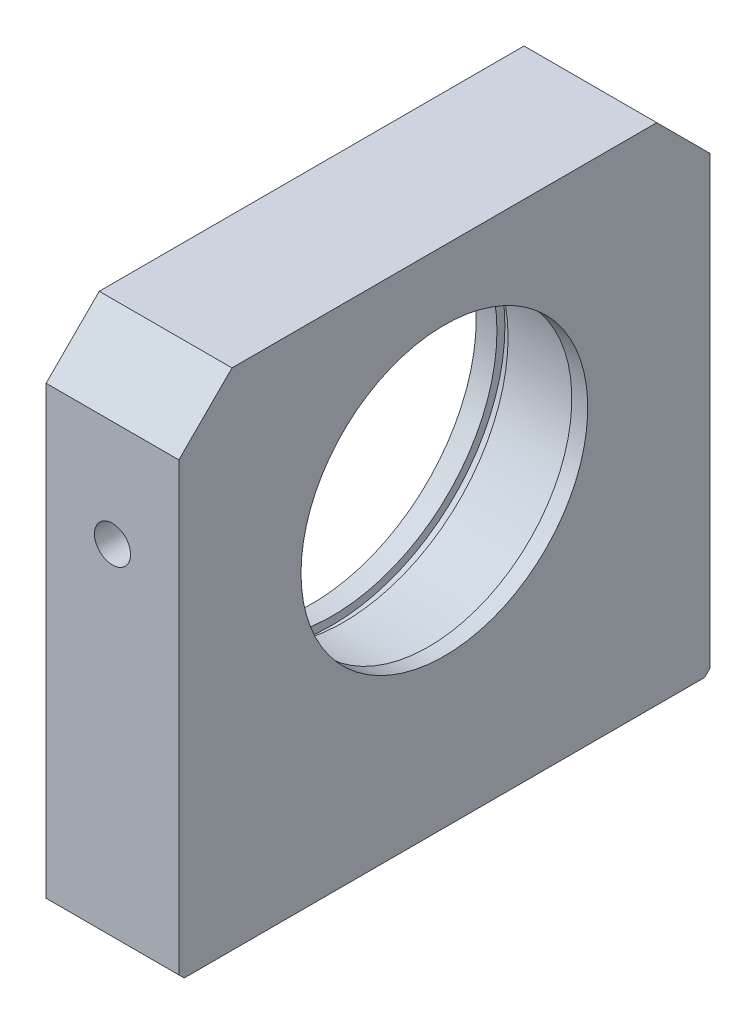
SolidWorks part; units mm, degrees
material "45#"
ref_plane "前基準面" through (0, 0, 0) normal (0, 0, 1) x (1, 0, 0)
ref_plane "上基準面" through (0, 0, 0) normal (0, 1, 0) x (1, 0, 0)
ref_plane "右基準面" through (0, 0, 0) normal (1, 0, 0) x (0, 0, -1)
sketch "草图1" plane through (0, 0, 0) normal (1, 0, 0) x (0, 0, -1)
  line L1 (-50, 47.5) -> (50, 47.5)
  line L2 (-50, 47.5) -> (-50, -47.5)
  line L3 (-50, -47.5) -> (50, -47.5)
  line L4 (50, 47.5) -> (50, -47.5)
  line L5 (-50, 47.5) -> (50, -47.5) construction
  line L6 (-50, -47.5) -> (50, 47.5) construction
  point P0 (0, 0)
  dimension "D1" = 95
  dimension "D2" = 100
extrude "凸台-拉伸1" add sketch "草图1" along normal blind 25
sketch "草图2" plane through (0, 0, 0) normal (-1, 0, 0) x (0, 0, 1)
  line L0 (0, 0) -> (0, 72.9224) construction
  line L1 (-50, 47.5) -> (50, 47.5) construction
  circle A0 centre (0, 7.5) radius 31
  dimension "D1" = 62
  dimension "D2" = 40
extrude "切除-拉伸1" cut sketch "草图2" against normal blind 22
sketch "草图3" plane through (22, 0, 0) normal (-1, 0, 0) x (0, 0, 1)
  circle A0 centre (0, 7.5) radius 27
  dimension "D1" = 54
extrude "切除-拉伸2" cut sketch "草图3" against normal through all
sketch "草图4" plane through (22, 0, 0) normal (-1, 0, 0) x (0, 0, 1)
  circle A0 centre (0, 7.5) radius 32.5
  dimension "D1" = 65
extrude "切除-拉伸3" cut sketch "草图4" along normal blind 2.1 from offset 16
hole_wizard "M8 螺纹孔1" positions "草图5" profile "草图6" tap size "M8" standard "GB"
sketch "草图5" plane through (0, 0, 50) normal (0, 0, 1) x (1, 0, 0)
  line L0 (12.5, 47.5) -> (12.5, -25.3343) construction
  line L1 (25, 47.5) -> (0, 47.5) construction
  point P0 (12.5, 17.5)
  dimension "D1" = 30
sketch "草图6" plane through (12.5, 17.5, 50) normal (1, 0, 0) x (0, -1, 0)
  line L0 (0, 0) -> (0, 17.7929)
  line L1 (0, 17.7929) -> (3.4, 15.75)
  line L2 (3.4, 15.75) -> (3.4, 0)
  line L5 (3.4, 0) -> (0, 0)
  line L10 (0, 17.7929) -> (-3.4, 15.75) construction
  line L11 (0, -6.35) -> (0, 107.95) construction
  dimension "螺纹孔钻头直径" = 6.8
  dimension "螺纹孔钻头深度" = 15.75
  dimension "导头角度" = 118
cosmetic thread "孔螺蚊线1" parameters "D1"=12, "D2"=8
hole_wizard "M8 螺纹孔2" positions "草图7" profile "草图8" tap size "M8" standard "GB"
sketch "草图7" plane through (0, 0, -50) normal (0, 0, -1) x (-1, 0, 0)
  point P0 (-12.5, 17.5)
sketch "草图8" plane through (12.5, 17.5, -50) normal (1, 0, 0) x (0, 1, 0)
  line L0 (0, 0) -> (0, 17.7929)
  line L1 (0, 17.7929) -> (3.4, 15.75)
  line L2 (3.4, 15.75) -> (3.4, 0)
  line L5 (3.4, 0) -> (0, 0)
  line L10 (0, 17.7929) -> (-3.4, 15.75) construction
  line L11 (0, -6.35) -> (0, 107.95) construction
  dimension "螺纹孔钻头直径" = 6.8
  dimension "螺纹孔钻头深度" = 15.75
  dimension "导头角度" = 118
cosmetic thread "孔螺蚊线2" parameters "D1"=12, "D2"=8
chamfer "倒角1" distance 10 angle 45 2 edges at (12.5, 47.5, -50) (12.5, 47.5, 50)
chamfer "倒角2" distance 1 angle 45 2 edges at (12.5, -47.5, -50) (12.5, -47.5, 50)
hole_wizard "M8 螺纹孔3" positions "草图9" profile "草图10" tap size "M8" standard "GB"
sketch "草图9" plane through (0, -47.5, 0) normal (0, -1, 0) x (-1, 0, 0)
  line L0 (0, 0) -> (-25, 0) construction
  line L1 (-25, -49) -> (-25, 49) construction
  point P0 (-12.5, -40)
  point P2 (-12.5, 0)
  point P12 (-12.5, 40)
  dimension "D1" = 80
sketch "草图10" plane through (12.5, -47.5, 40) normal (1, 0, 0) x (0, 0, -1)
  line L0 (0, 0) -> (0, 21.7929)
  line L1 (0, 21.7929) -> (3.4, 19.75)
  line L2 (3.4, 19.75) -> (3.4, 0)
  line L5 (3.4, 0) -> (0, 0)
  line L10 (0, 21.7929) -> (-3.4, 19.75) construction
  line L11 (0, -6.35) -> (0, 107.95) construction
  dimension "螺纹孔钻头直径" = 6.8
  dimension "螺纹孔钻头深度" = 19.75
  dimension "导头角度" = 118
cosmetic thread "孔螺蚊线3" parameters "D1"=16, "D2"=8
cosmetic thread "孔螺蚊线4" parameters "D1"=16, "D2"=8
cosmetic thread "孔螺蚊线5" parameters "D1"=16, "D2"=8
